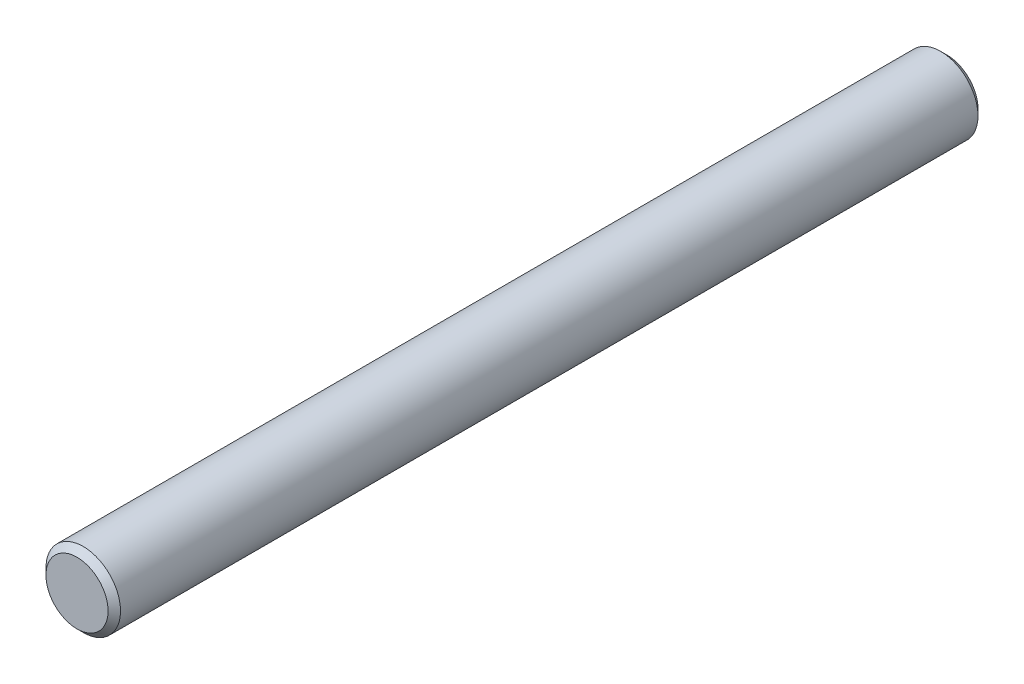
SolidWorks part; units mm, degrees
ref_plane "Front Plane" through (0, 0, 0) normal (0, 0, 1) x (1, 0, 0)
ref_plane "Top Plane" through (0, 0, 0) normal (0, 1, 0) x (1, 0, 0)
ref_plane "Right Plane" through (0, 0, 0) normal (1, 0, 0) x (0, 0, -1)
sketch "Sketch1" plane through (0, 0, 0) normal (0, 0, 1) x (1, 0, 0)
  circle A0 centre (81.0002, -185.4519) radius 3
extrude "Boss-Extrude1" add sketch "Sketch1" against normal blind 70
chamfer "Chamfer1" distance 0.5 angle 45 2 edges at (84.0002, -185.4519, -70) (84.0002, -185.4519, 0)
